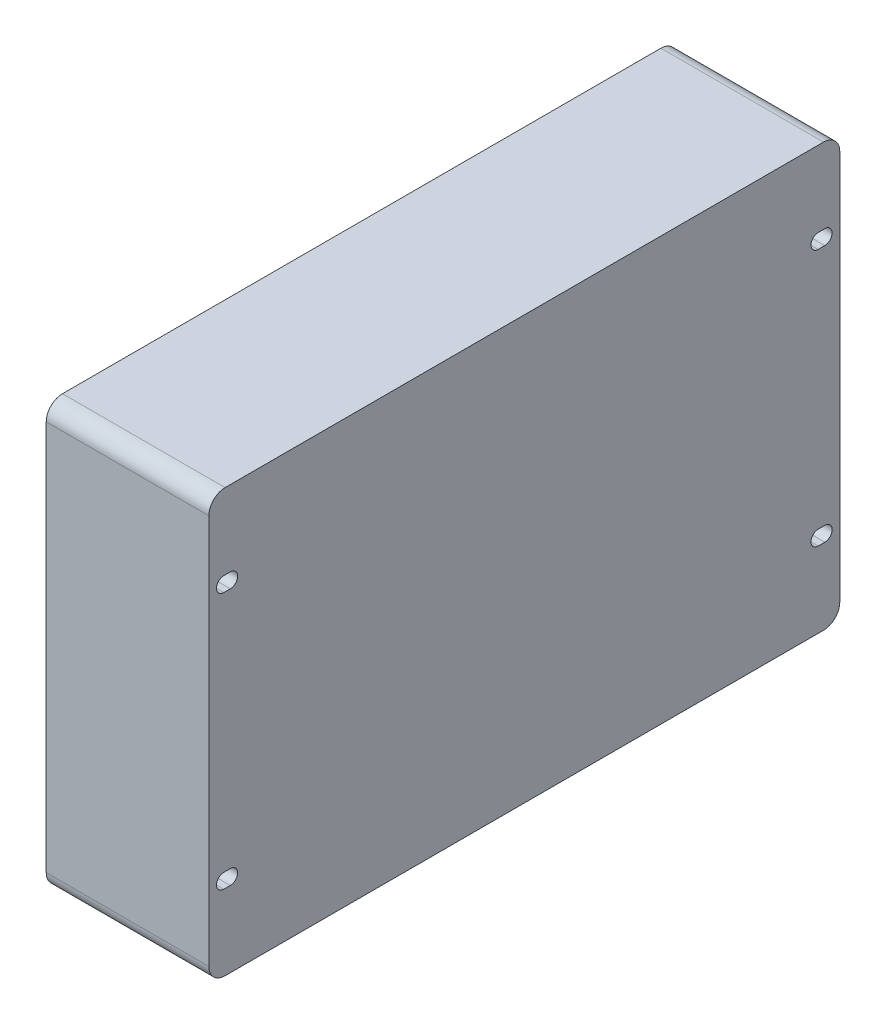
SolidWorks part; units mm, degrees
material "SPCC冷轧板喷塑"
ref_plane "前视基准面" through (0, 0, 0) normal (0, 0, 1) x (1, 0, 0)
ref_plane "上视基准面" through (0, 0, 0) normal (0, 1, 0) x (1, 0, 0)
ref_plane "右视基准面" through (0, 0, 0) normal (1, 0, 0) x (0, 0, -1)
other "Configuration Table"
sketch "草图1" plane through (0, 0, 0) normal (1, 0, 0) x (0, 0, -1)
  line L1 (194, -130) -> (-194, -130)
  line L2 (194, -130) -> (194, 130)
  line L3 (194, 130) -> (-194, 130)
  line L4 (-194, -130) -> (-194, 130)
  line L5 (194, -130) -> (-194, 130) construction
  line L6 (194, 130) -> (-194, -130) construction
  point P0 (0, 0)
  dimension "D1" = 388
  dimension "D2" = 260
extrude "凸台-拉伸1" add sketch "草图1" along normal mid plane 100
sketch "草图2" plane through (50, 0, 0) normal (1, 0, 0) x (0, 0, -1)
  line L0 (-184.8, 79) -> (-180.8, 79) construction
  line L1 (-184.8, 83.5) -> (-180.8, 83.5)
  line L2 (-184.8, 74.5) -> (-180.8, 74.5)
  line L3 (180.8, 79) -> (184.8, 79) construction
  line L4 (180.8, 83.5) -> (184.8, 83.5)
  line L5 (180.8, 74.5) -> (184.8, 74.5)
  line L6 (180.8, -79) -> (184.8, -79) construction
  line L7 (180.8, -74.5) -> (184.8, -74.5)
  line L8 (180.8, -83.5) -> (184.8, -83.5)
  line L9 (-184.8, -79) -> (-180.8, -79) construction
  line L10 (-184.8, -74.5) -> (-180.8, -74.5)
  line L11 (-184.8, -83.5) -> (-180.8, -83.5)
  line L12 (-184.8, 79) -> (180.8, 79) construction
  line L13 (-184.8, 79) -> (-184.8, -79) construction
  arc A0 (-184.8, 83.5) -> (-184.8, 74.5) centre (-184.8, 79) ccw
  arc A1 (-180.8, 74.5) -> (-180.8, 83.5) centre (-180.8, 79) ccw
  arc A2 (180.8, 83.5) -> (180.8, 74.5) centre (180.8, 79) ccw
  arc A3 (184.8, 74.5) -> (184.8, 83.5) centre (184.8, 79) ccw
  arc A4 (180.8, -74.5) -> (180.8, -83.5) centre (180.8, -79) ccw
  arc A5 (184.8, -83.5) -> (184.8, -74.5) centre (184.8, -79) ccw
  arc A6 (-184.8, -74.5) -> (-184.8, -83.5) centre (-184.8, -79) ccw
  arc A7 (-180.8, -83.5) -> (-180.8, -74.5) centre (-180.8, -79) ccw
  point P2 (-182.8, 79)
  point P13 (182.8, 79)
  point P20 (182.8, -79)
  point P27 (-182.8, -79)
  dimension "D2" = 13
  dimension "D1" = 9
  dimension "D3" = 79
  dimension "D4" = 182.8
  dimension "D7" = 365.6
  dimension "D8" = 158
  dimension "D5" = 2
  dimension "D6" = 2
extrude "切除-拉伸1" cut sketch "草图2" against normal blind 100
fillet "圆角1" radius 10 4 edges at (0, 130, -194) (0, -130, -194) (0, -130, 194) (0, 130, 194)
